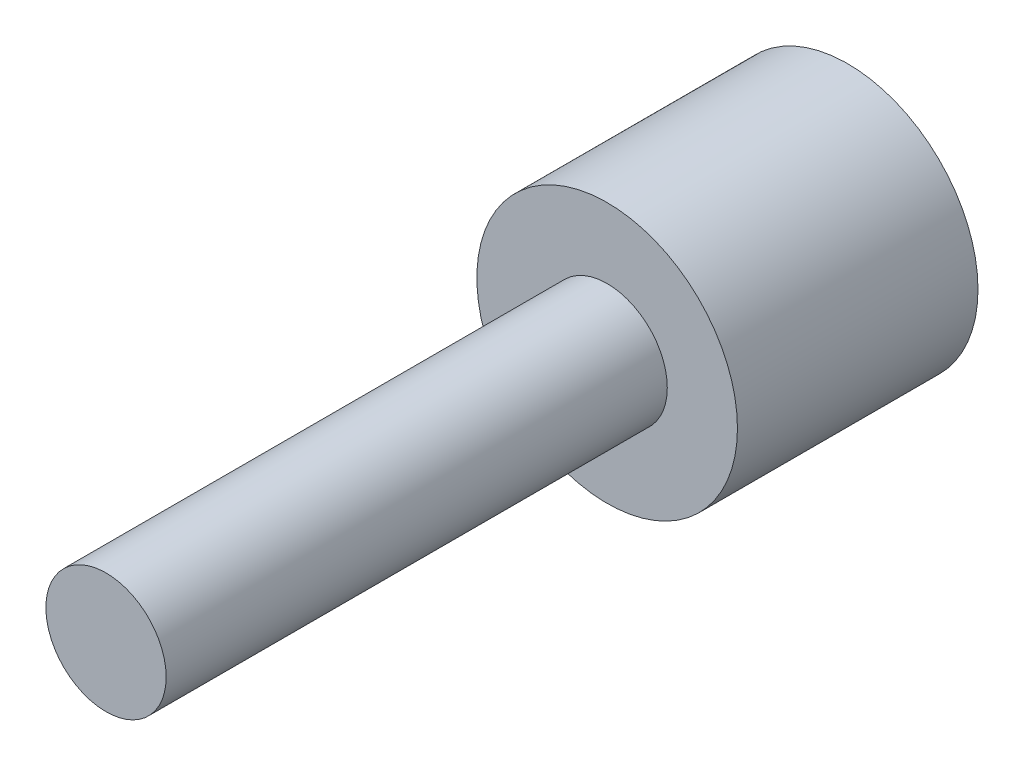
from build123d import *

# Parameters (mm, degrees)
SKETCH_1_R          = 6.5
EXTRUDE_1_DEPTH     = 12
SKETCH_2_R          = 3
EXTRUDE_2_DEPTH     = 25
SKETCH_3_R          = 5
CUT_EXTRUDE_1_DEPTH = 0.5


with BuildPart() as part:
    # 草图1 → 凸台-拉伸1 (new body)
    with BuildSketch(Plane.XY):
        Circle(SKETCH_1_R)
    extrude(amount=EXTRUDE_1_DEPTH)

    # 草图2 → 凸台-拉伸2 (add)
    with BuildSketch(Plane.XY.offset(12)):
        Circle(SKETCH_2_R)
    extrude(amount=EXTRUDE_2_DEPTH)

    # 草图3 → 切除-拉伸1 (cut)
    with BuildSketch(Plane(origin=(0, 0, 0), x_dir=(-1, 0, 0), z_dir=(0, 0, -1))):
        Circle(SKETCH_3_R)
    extrude(amount=-CUT_EXTRUDE_1_DEPTH, mode=Mode.SUBTRACT)


solid = part.part
